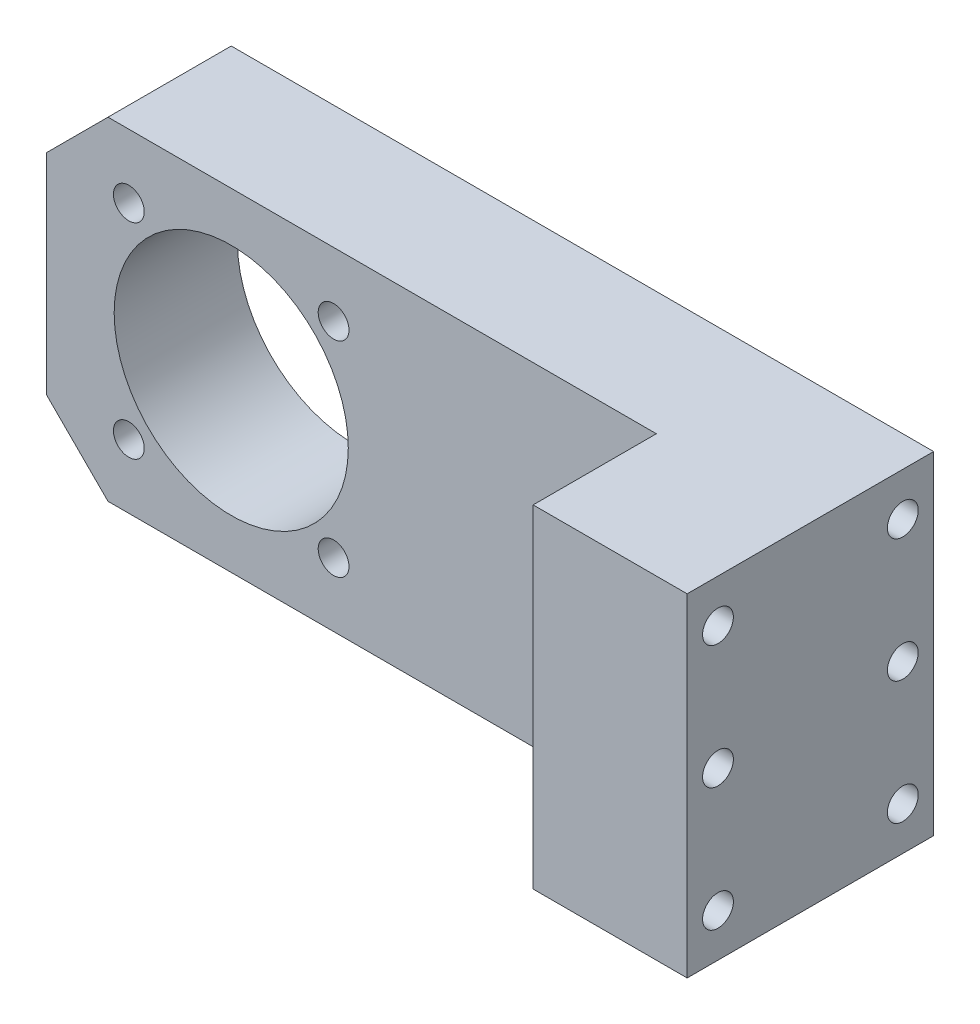
from build123d import *

# Parameters (mm, degrees)
SKETCH1_W             = 124
SKETCH1_H             = 54
BOSS_EXTRUDE1_DEPTH   = 20
CHAMFER1_SIZE         = 10
SKETCH2_R             = 19
CUT_EXTRUDE1_DEPTH    = 20
M6_TAPPED_HOLE1_D     = 5
CIRPATTERN1_COUNT     = 4
SKETCH7_W             = 25
SKETCH7_H             = 54
BOSS_EXTRUDE2_DEPTH   = 20
M6_TAPPED_HOLE2_D     = 5
M6_TAPPED_HOLE2_DEPTH = 15
M6_TAPPED_HOLE2_TIP   = 1.502151548


with BuildPart() as part:
    # Sketch1 → Boss-Extrude1 (new body)
    with BuildSketch(Plane.XY):
        with Locations((62, 27)):
            Rectangle(SKETCH1_W, SKETCH1_H)
    extrude(amount=BOSS_EXTRUDE1_DEPTH)

    # Chamfer1
    chamfer1_edges = [part.edges().sort_by_distance(p)[0] for p in [
        (0, 54, 10),
        (0, 0, 10),
    ]]
    chamfer(chamfer1_edges, length=CHAMFER1_SIZE)

    # Sketch2 → Cut-Extrude1 (cut)
    with BuildSketch(Plane.XY.offset(20)):
        with Locations((30, 27)):
            Circle(SKETCH2_R)
    extrude(amount=-CUT_EXTRUDE1_DEPTH, mode=Mode.SUBTRACT)

    # M6 Tapped Hole1 (through all)
    with Locations(Plane.XY.offset(20)):
        with Locations((46.617009358, 43.617009358)):
            m6_tapped_hole1 = Hole(M6_TAPPED_HOLE1_D / 2)

    # CirPattern1: M6 Tapped Hole1 ×4 about axis
    cirpattern1_axis = Axis((30, 27, 0), (0, 0, 1))
    for i in range(1, CIRPATTERN1_COUNT):
        add(m6_tapped_hole1.rotate(cirpattern1_axis, i * 360 / CIRPATTERN1_COUNT), mode=Mode.SUBTRACT)

    # Sketch7 → Boss-Extrude2 (add)
    with BuildSketch(Plane.XY.offset(20)):
        with Locations((111.5, 27)):
            Rectangle(SKETCH7_W, SKETCH7_H)
    extrude(amount=BOSS_EXTRUDE2_DEPTH)

    # M6 Tapped Hole2
    with Locations(Plane(origin=(124, 0, 0), x_dir=(0, 0, -1), z_dir=(1, 0, 0))):
        with Locations((-35, 47), (-5, 47), (-35, 7), (-5, 7), (-35, 27), (-5, 27)):
            Hole(M6_TAPPED_HOLE2_D / 2, depth=M6_TAPPED_HOLE2_DEPTH)
            with Locations((0, 0, -(M6_TAPPED_HOLE2_DEPTH + M6_TAPPED_HOLE2_TIP / 2))):  # 118° drill point
                Cone(0, M6_TAPPED_HOLE2_D / 2, M6_TAPPED_HOLE2_TIP, mode=Mode.SUBTRACT)


solid = part.part
